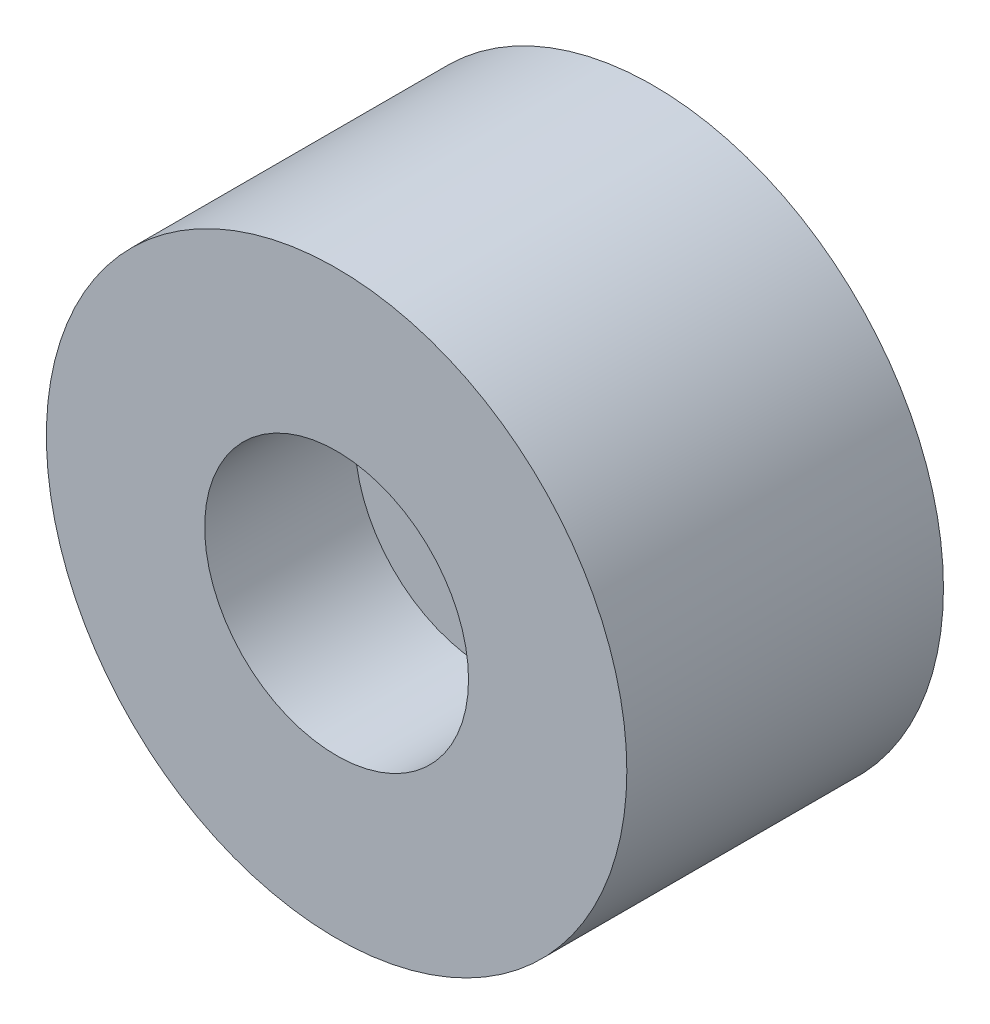
from build123d import *

# Parameters (mm, degrees)
SKETCH_1_R                = 11
EXTRUDE_1_DEPTH           = 12
HOLE_WIZARD_1_D           = 5.5
HOLE_WIZARD_1_CBORE_D     = 10
HOLE_WIZARD_1_CBORE_DEPTH = 5.7


with BuildPart() as part:
    # 草图1 → 凸台-拉伸1 (new body)
    with BuildSketch(Plane.XY):
        Circle(SKETCH_1_R)
    extrude(amount=EXTRUDE_1_DEPTH)

    # 打孔尺寸(%根据)内六角圆柱头螺钉的类型1 (through all)
    with Locations(Plane.XY.offset(12)):
        with Locations((0, 0)):
            CounterBoreHole(HOLE_WIZARD_1_D / 2, HOLE_WIZARD_1_CBORE_D / 2, HOLE_WIZARD_1_CBORE_DEPTH)


solid = part.part
